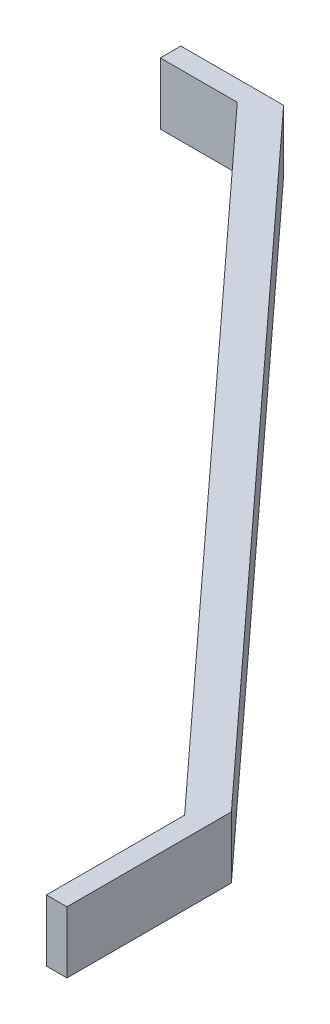
from build123d import *

# Parameters (mm, degrees)
BOSS_EXTRUDE1_DEPTH = 15


with BuildPart() as part:
    # Sketch1 → Boss-Extrude1 (new body)
    with BuildSketch(Plane.XZ.offset(-500)):
        Polygon((376.666458359, 456.299687539), (376.666458359, 416.299687539), (234.166458359, 261.099687539), (209.166458359, 261.099687539), (209.166458359, 266.099687539), (227.89663092, 266.099687539), (361.870871539, 412.014088551), (371.666458359, 422.682685565), (371.666458359, 456.299687539), align=None)
    extrude(amount=-BOSS_EXTRUDE1_DEPTH)


solid = part.part
